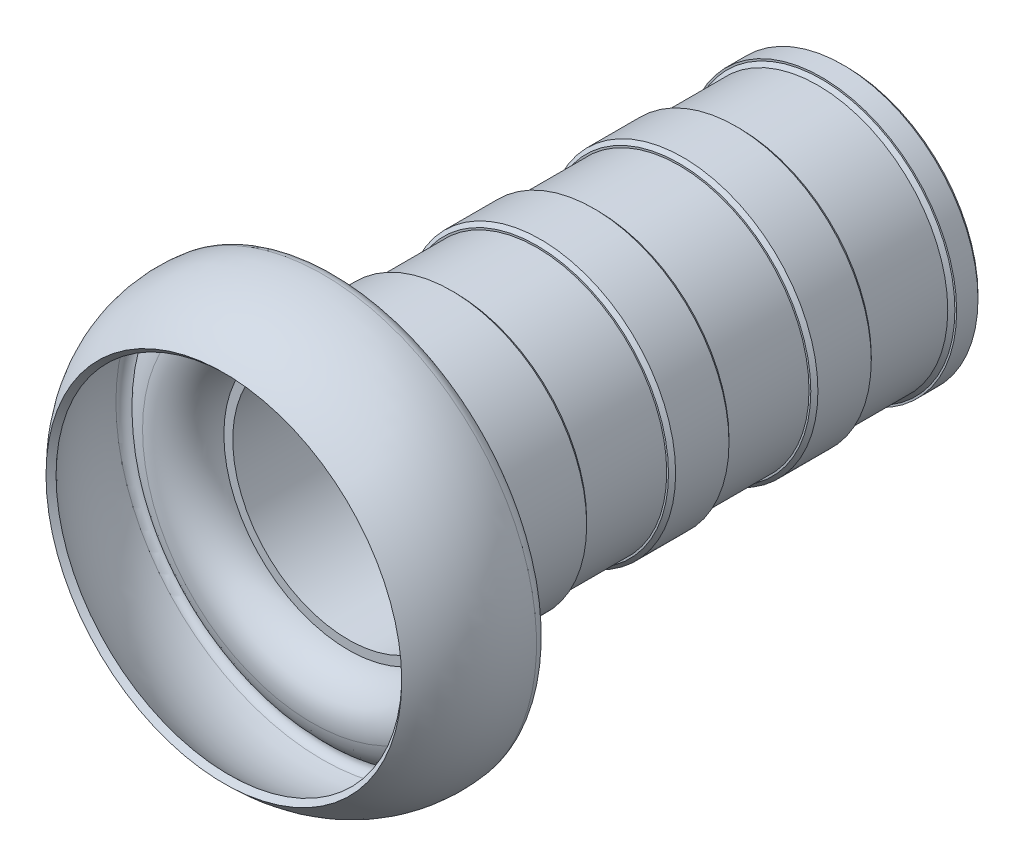
from build123d import *

# Parameters (mm, degrees)
SKETCH_1_R             = 38
SKETCH_1_R_2           = 32.5
EXTRUDE_1_DEPTH        = 140
CHAMFER_1_SIZE         = 1
CUT_EXTRUDE_START      = -23
SKETCH_2_R             = 38
SKETCH_2_R_2           = 36.5
CUT_EXTRUDE_1_DEPTH    = 23
PATTERN_LINEAR_1_COUNT = 3
PATTERN_LINEAR_1_PITCH = 40
CHAMFER_2_SIZE         = 1


with BuildPart() as part:
    # 草图1 → 凸台-拉伸1 (new body)
    with BuildSketch(Plane.XY):
        Circle(SKETCH_1_R)
        Circle(SKETCH_1_R_2, mode=Mode.SUBTRACT)
    extrude(amount=EXTRUDE_1_DEPTH)

    # 倒角1
    chamfer_1_edges = [part.edges().sort_by_distance(p)[0] for p in [
        (-38, 0, 140),
    ]]
    chamfer(chamfer_1_edges, length=CHAMFER_1_SIZE)

    # 草图2 → 切除-拉伸1 (cut)
    with BuildSketch(Plane.XY.offset(110).offset(CUT_EXTRUDE_START)):
        Circle(SKETCH_2_R)
        Circle(SKETCH_2_R_2, mode=Mode.SUBTRACT)
    cut_extrude_1 = extrude(amount=CUT_EXTRUDE_1_DEPTH, mode=Mode.SUBTRACT)

    # 阵列(线性)1: 切除-拉伸1 ×3
    with Locations(*[(0, 0, -i * PATTERN_LINEAR_1_PITCH) for i in range(1, PATTERN_LINEAR_1_COUNT)]):
        add(cut_extrude_1, mode=Mode.SUBTRACT)

    # 倒角2
    chamfer_2_edges = [part.edges().sort_by_distance(p)[0] for p in [
        (-38, 0, 87),
        (-38, 0, 110),
        (-38, 0, 0),
        (-38, 0, 47),
        (-38, 0, 70),
        (-36.5, 0, 7),
        (-38, 0, 30),
    ]]
    chamfer(chamfer_2_edges, length=CHAMFER_2_SIZE)

    # 草图3 → 旋转1 (revolve)
    with BuildSketch(Plane(origin=(0, 0, 0), x_dir=(1, 0, 0), z_dir=(0, 1, 0)), mode=Mode.PRIVATE) as revolve_1_sk:
        with BuildLine():
            Line((50, -175), (48.614771624, -173.557383507))
            ThreePointArc((48.614771624, -173.557383507), (56.395121663, -161.54929973), (58.013767993, -147.332833686))
            ThreePointArc((58.013767993, -147.332833686), (57.136760156, -145.772105393), (55.411246429, -145.295012185))
            ThreePointArc((55.411246429, -145.295012185), (51.963704542, -148.463135482), (47.627927509, -150.230502962))
            ThreePointArc((47.627927509, -150.230502962), (38.874805833, -148.126003692), (35, -140))
            Line((35, -140), (37, -140))
            ThreePointArc((37, -140), (40.133789135, -146.571989199), (47.212966464, -148.274024664))
            ThreePointArc((47.212966464, -148.274024664), (51.171077472, -146.59169845), (54.205200918, -143.543590978))
            ThreePointArc((54.205200918, -143.543590978), (57.964649, -143.915891309), (60, -147.098563727))
            ThreePointArc((60, -147.098563727), (58.277851947, -162.224078714), (50, -175))
        make_face()
    revolve(revolve_1_sk.sketch.rotate(Axis((0, 0, 140), (0, 0, 1)), 180), axis=Axis((0, 0, 140), (0, 0, 1)))


solid = part.part
